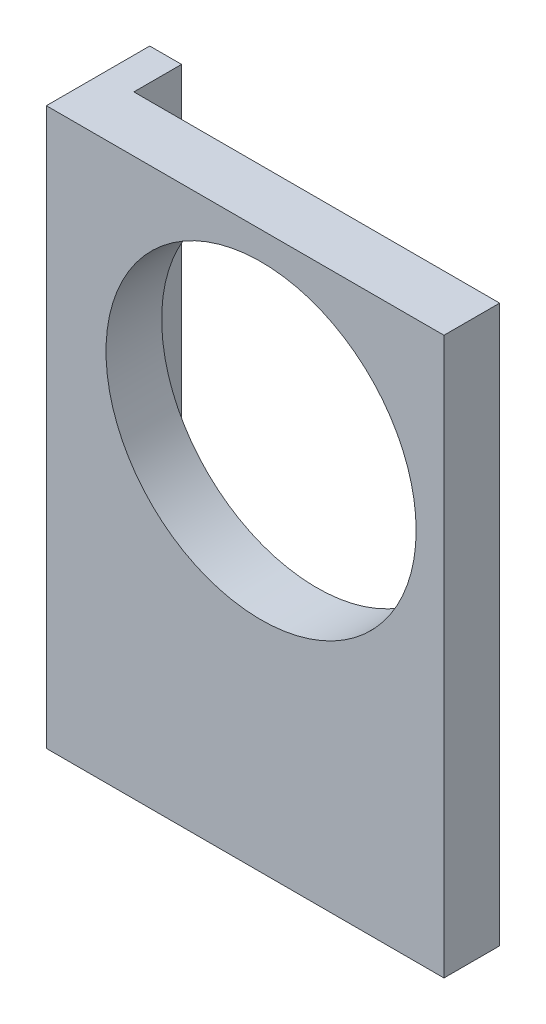
from build123d import *

# Parameters (mm, degrees)
SKETCH_1_W          = 100
SKETCH_1_H          = 140
EXTRUDE_1_DEPTH     = 14
CUT_EXTRUDE_1_REACH = 89.155
SKETCH_2_R          = 39
SKETCH_3_W          = 8
SKETCH_3_H          = 140
EXTRUDE_2_DEPTH     = 12


with BuildPart() as part:
    # 草图1 → 凸台-拉伸1 (new body)
    with BuildSketch(Plane.XY):
        Rectangle(SKETCH_1_W, SKETCH_1_H)
    extrude(amount=EXTRUDE_1_DEPTH)

    # 草图2 → 切除-拉伸1 (cut, up to next)
    with BuildSketch(Plane.XY.offset(14), mode=Mode.PRIVATE) as cut_extrude_1_sk1:
        with Locations((4, 24)):
            Circle(SKETCH_2_R)
    cut_extrude_1_tool1 = extrude(cut_extrude_1_sk1.sketch, amount=-CUT_EXTRUDE_1_REACH, mode=Mode.PRIVATE) & part.part
    add(cut_extrude_1_tool1.solids().sort_by_distance((4, 24, 14))[0], mode=Mode.SUBTRACT)

    # 草图3 → 凸台-拉伸2 (add)
    with BuildSketch(Plane.XY):
        with Locations((-46, 0)):
            Rectangle(SKETCH_3_W, SKETCH_3_H)
    extrude(amount=-EXTRUDE_2_DEPTH)


solid = part.part
